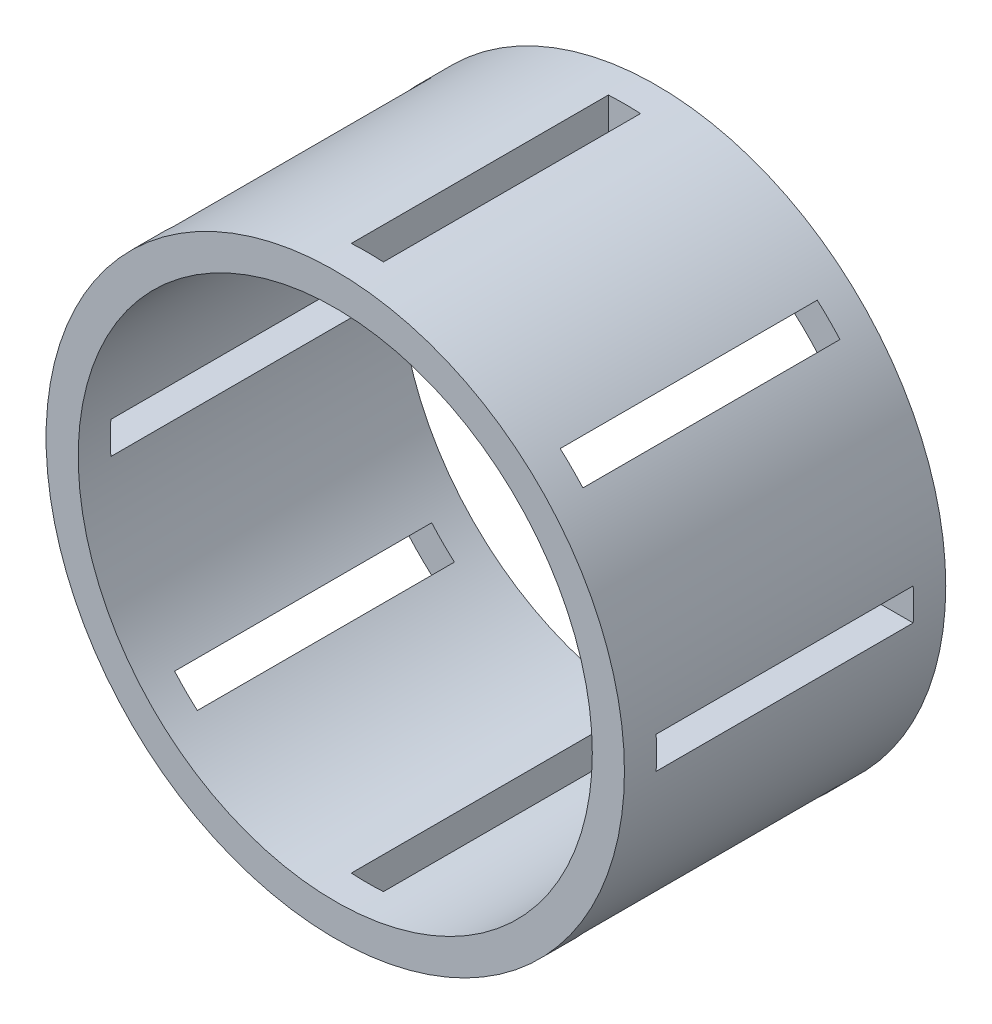
SolidWorks part; units mm, degrees
ref_plane "Front Plane" through (0, 0, 0) normal (0, 0, 1) x (1, 0, 0)
ref_plane "Top Plane" through (0, 0, 0) normal (0, 1, 0) x (1, 0, 0)
ref_plane "Right Plane" through (0, 0, 0) normal (1, 0, 0) x (0, 0, -1)
other "Configuration Table"
sketch "Sketch1" plane through (0, 0, 0) normal (0, 0, 1) x (1, 0, 0)
  circle A0 centre (-599.8842, -90) radius 45
  circle A1 centre (-599.8842, -90) radius 40
  dimension "D1" = 90
  dimension "D2" = 80
extrude "Boss-Extrude1" add sketch "Sketch1" along normal blind 50
sketch "Sketch2" plane through (0, 0, 0) normal (0, 1, 0) x (1, 0, 0)
  line L0 (-599.8842, -50) -> (-599.8842, 0) construction
  line L1 (-602.3842, -45) -> (-597.3842, -45)
  line L2 (-602.3842, -45) -> (-602.3842, -5)
  line L3 (-602.3842, -5) -> (-597.3842, -5)
  line L4 (-597.3842, -45) -> (-597.3842, -5)
  line L5 (-602.3842, -45) -> (-597.3842, -5) construction
  line L6 (-602.3842, -5) -> (-597.3842, -45) construction
  point P0 (-599.8842, -25)
  dimension "D1" = 40
  dimension "D2" = 5
extrude "Cut-Extrude1" cut sketch "Sketch2" against normal through all both and the other way through all
pattern_circular "CirPattern1" count 8 over 360 about axis through (-599.8842, -90, 0) along (0, 0, 1) of "Cut-Extrude1"
